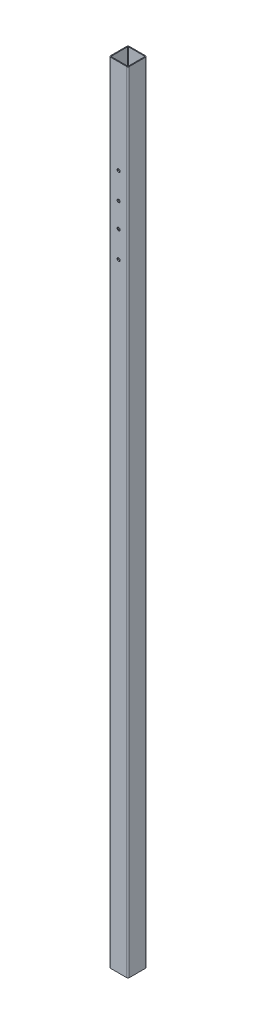
from build123d import *

# Parameters (mm, degrees)
BOSS_EXTRUDE1_DEPTH     = 2097
CUT_EXTRUDE1_DEPTH      = 2098.744979734
CUT_EXTRUDE1_DEPTH_BACK = 2098.744979734
SKETCH2_R               = 4


with BuildPart() as part:
    # Sketch1 → Boss-Extrude1 (new body)
    with BuildSketch(Plane(origin=(0, 0, 0), x_dir=(1, 0, 0), z_dir=(0, 1, 0))):
        with BuildLine():
            Line((-21.55, -25), (21.55, -25))
            ThreePointArc((21.55, -25), (23.989518395, -23.989518395), (25, -21.55))
            Line((25, -21.55), (25, 21.55))
            ThreePointArc((25, 21.55), (23.989518395, 23.989518395), (21.55, 25))
            Line((21.55, 25), (-21.55, 25))
            ThreePointArc((-21.55, 25), (-23.989518395, 23.989518395), (-25, 21.55))
            Line((-25, 21.55), (-25, -21.55))
            ThreePointArc((-25, -21.55), (-23.989518395, -23.989518395), (-21.55, -25))
        make_face()
        with BuildLine():
            Line((-21.55, -22.7), (21.55, -22.7))
            ThreePointArc((21.55, -22.7), (22.363172798, -22.363172798), (22.7, -21.55))
            Line((22.7, -21.55), (22.7, 21.55))
            ThreePointArc((22.7, 21.55), (22.363172798, 22.363172798), (21.55, 22.7))
            Line((21.55, 22.7), (-21.55, 22.7))
            ThreePointArc((-21.55, 22.7), (-22.363172798, 22.363172798), (-22.7, 21.55))
            Line((-22.7, 21.55), (-22.7, -21.55))
            ThreePointArc((-22.7, -21.55), (-22.363172798, -22.363172798), (-21.55, -22.7))
        make_face(mode=Mode.SUBTRACT)
    extrude(amount=BOSS_EXTRUDE1_DEPTH)

    # Sketch2 → Cut-Extrude1 (cut, two sides: drawn at the far end of the back side and taken through both)
    with BuildSketch(Plane(origin=(0, 0, -25), x_dir=(-1, 0, 0), z_dir=(0, 0, -1)).offset(-CUT_EXTRUDE1_DEPTH_BACK)):
        with Locations(Location((0, 1847, 0), (0, 0, 180))):
            Circle(SKETCH2_R)
        with Locations(Location((0, 1777, 0), (0, 0, 180))):
            Circle(SKETCH2_R)
        with Locations(Location((0, 1712, 0), (0, 0, 180))):
            Circle(SKETCH2_R)
        with Locations(Location((0, 1642, 0), (0, 0, 180))):
            Circle(SKETCH2_R)
    extrude(amount=CUT_EXTRUDE1_DEPTH + CUT_EXTRUDE1_DEPTH_BACK, mode=Mode.SUBTRACT)


solid = part.part
